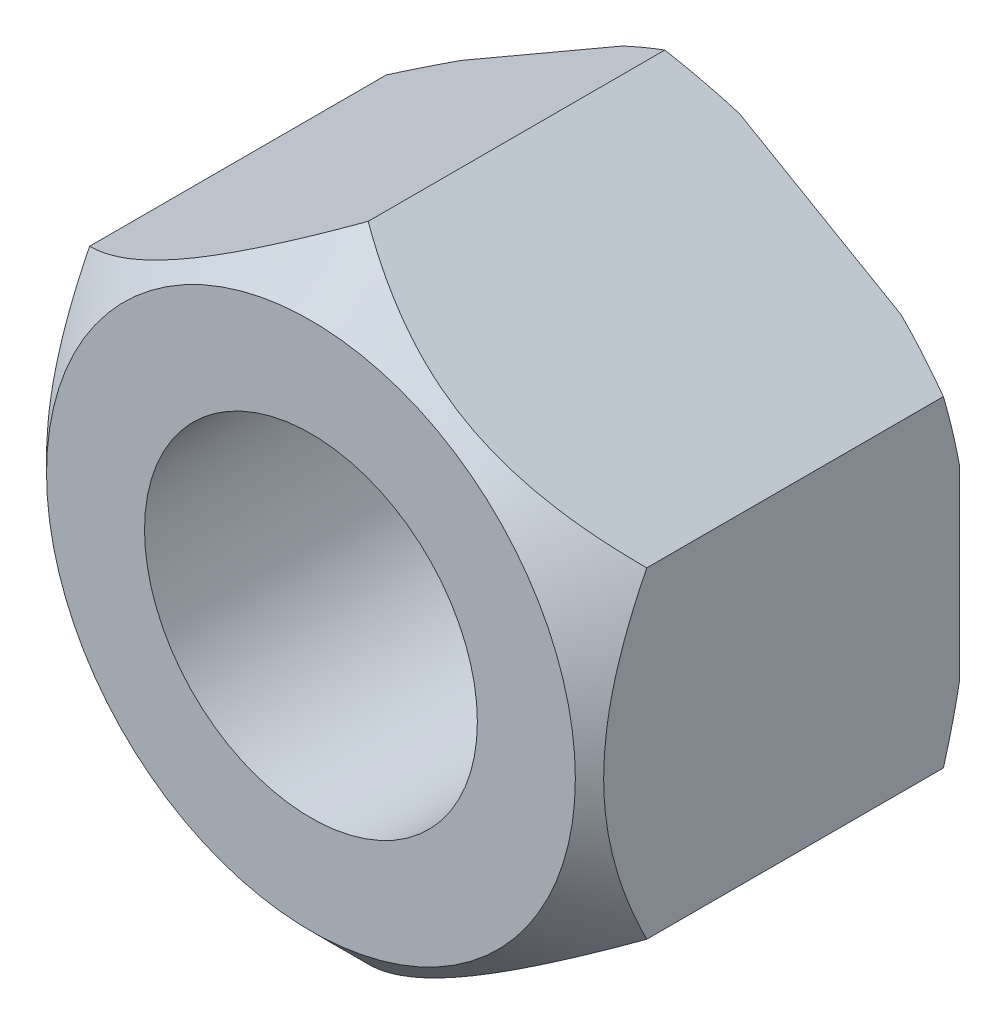
from build123d import *

# Parameters (mm, degrees)
SKETCH_1_R          = 7.646875
EXTRUDE_555_DEPTH   = 17
SKETCH_2_OUTSIDE_W  = 129.344
SKETCH_2_OUTSIDE_H  = 133.304
SKETCH_2_OUTSIDE_R  = 13.5
CUT_EXTRUDE_1_DEPTH = 26.909162472
CUT_EXTRUDE_1_DRAFT = -60
CHAMFER_1_SIZE      = 0.294642857
SKETCH_9_OUTSIDE_W  = 89.946
SKETCH_9_OUTSIDE_H  = 93.906
SKETCH_9_OUTSIDE_R  = 12.15
CUT_EXTRUDE_7_DEPTH = 26.909162472
CUT_EXTRUDE_7_DRAFT = -45


with BuildPart() as part:
    # 草图1 → Extrude 555 (new body)
    with BuildSketch(Plane.XY):
        Polygon((0, 14.78), (-12.799855468, 7.39), (-12.799855468, -7.39), (0, -14.78), (12.799855468, -7.39), (12.799855468, 7.39), align=None)
        Circle(SKETCH_1_R, mode=Mode.SUBTRACT)
    extrude(amount=EXTRUDE_555_DEPTH)


with BuildPart() as cut_extrude_1_tool:
    # 草图2 outside → 切除-拉伸1 (with draft: the straight prism first)
    with BuildSketch(Plane(origin=(0, 0, 0), x_dir=(-1, 0, 0), z_dir=(0, 0, -1))):
        Rectangle(SKETCH_2_OUTSIDE_W, SKETCH_2_OUTSIDE_H)
        Circle(SKETCH_2_OUTSIDE_R, mode=Mode.SUBTRACT)
    extrude(amount=-CUT_EXTRUDE_1_DEPTH)
    # 切除-拉伸1: the draft: its side faces are tilted about the plane it starts from
    cut_extrude_1_sides = [cut_extrude_1_tool.faces().sort_by_distance(p)[0] for p in [
        (0, -66.652, 13.454581236),
        (-64.672, 0, 13.454581236),
        (0, 66.652, 13.454581236),
        (64.672, 0, 13.454581236),
        (13.5, 0, 13.454581236),
    ]]
    draft(cut_extrude_1_sides, Plane(origin=(0, 0, 0), x_dir=(-1, 0, 0), z_dir=(0, 0, -1)), CUT_EXTRUDE_1_DRAFT)


with BuildPart() as part_1:
    add(part.part)

    # 切除-拉伸1: cut by cut_extrude_1_tool
    add(cut_extrude_1_tool.part, mode=Mode.SUBTRACT)

    # 倒角1
    chamfer_1_edges = [part_1.edges().sort_by_distance(p)[0] for p in [
        (-7.646875, 0, 0),
    ]]
    chamfer(chamfer_1_edges, length=CHAMFER_1_SIZE)


with BuildPart() as cut_extrude_7_tool:
    # 草图9 outside → 切除-拉伸7 (with draft: the straight prism first)
    with BuildSketch(Plane.XY.offset(17)):
        Rectangle(SKETCH_9_OUTSIDE_W, SKETCH_9_OUTSIDE_H)
        Circle(SKETCH_9_OUTSIDE_R, mode=Mode.SUBTRACT)
    extrude(amount=-CUT_EXTRUDE_7_DEPTH)
    # 切除-拉伸7: the draft: its side faces are tilted about the plane it starts from
    cut_extrude_7_sides = [cut_extrude_7_tool.faces().sort_by_distance(p)[0] for p in [
        (0, -46.953, 3.545418764),
        (44.973, 0, 3.545418764),
        (0, 46.953, 3.545418764),
        (-44.973, 0, 3.545418764),
        (-12.15, 0, 3.545418764),
    ]]
    draft(cut_extrude_7_sides, Plane.XY.offset(17), CUT_EXTRUDE_7_DRAFT)


with BuildPart() as part_2:
    add(part_1.part)

    # 切除-拉伸7: cut by cut_extrude_7_tool
    add(cut_extrude_7_tool.part, mode=Mode.SUBTRACT)


solid = part_2.part
